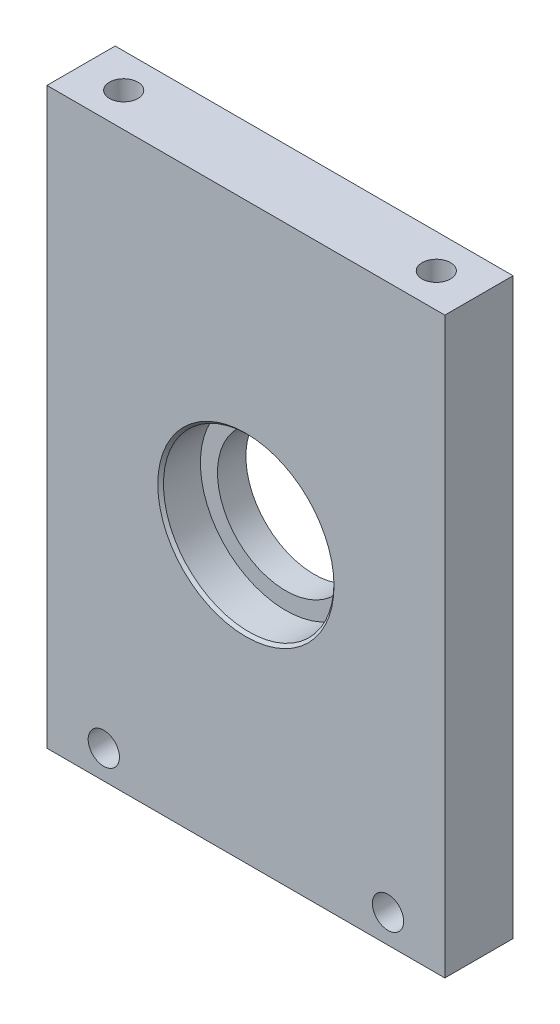
SolidWorks part; units mm, degrees
ref_plane "前视" through (0, 0, 0) normal (0, 0, 1) x (1, 0, 0)
ref_plane "上视" through (0, 0, 0) normal (0, 1, 0) x (1, 0, 0)
ref_plane "右视" through (0, 0, 0) normal (1, 0, 0) x (0, 0, -1)
sketch "草图1" plane through (0, 0, 0) normal (0, 0, 1) x (1, 0, 0)
  line L1 (0, 0) -> (70, 0)
  line L2 (0, 0) -> (0, -101)
  line L3 (0, -101) -> (70, -101)
  line L4 (70, 0) -> (70, -101)
  dimension "D1" = 70
  dimension "D2" = 101
extrude "凸台-拉伸1" add sketch "草图1" along normal blind 12
sketch "草图2" plane through (0, 0, 12) normal (0, 0, 1) x (1, 0, 0)
  line L0 (35, -51) -> (35, -101) construction
  line L1 (0, -101) -> (70, -101) construction
  circle A0 centre (35, -51) radius 15
  dimension "D1" = 30
  dimension "D2" = 50
extrude "切除-拉伸1" cut sketch "草图2" against normal blind 7
sketch "草图3" plane through (0, 0, 5) normal (0, 0, 1) x (1, 0, 0)
  circle A0 centre (35, -51) radius 12
  dimension "D1" = 24
extrude "切除-拉伸2" cut sketch "草图3" against normal through all
chamfer "倒角2" distance 0.5 angle 45 1 edges at (50, -51, 12)
hole_wizard "M6 螺纹孔1" positions "草图5" profile "草图4" tap size "M6" standard "GB"
sketch "草图5" plane through (0, 0, 0) normal (0, 1, 0) x (1, 0, 0)
  line L0 (62.5, -6) -> (7.5, -6) construction
  line L3 (35, -6) -> (35, -12) construction
  line L4 (70, -12) -> (0, -12) construction
  point P0 (62.5, -6)
  point P2 (7.5, -6)
  dimension "D1" = 6
  dimension "D2" = 55
sketch "草图4" plane through (62.5, 0, 6) normal (1, 0, 0) x (0, 0, 1)
  line L0 (0, 0) -> (0, 18.5022)
  line L1 (0, 18.5022) -> (2.5, 17)
  line L2 (2.5, 17) -> (2.5, 0)
  line L5 (2.5, 0) -> (0, 0)
  line L10 (0, 18.5022) -> (-2.5, 17) construction
  line L11 (0, -6.35) -> (0, 107.95) construction
  dimension "螺纹孔钻头直径" = 5
  dimension "螺纹孔钻头深度" = 17
  dimension "导头角度" = 118
cosmetic thread "孔螺蚊线1" parameters "D1"=12, "D2"=6
cosmetic thread "孔螺蚊线2" parameters "D1"=12, "D2"=6
sketch "草图10" plane through (0, 0, 0) normal (0, 0, -1) x (-1, 0, 0)
  line L0 (-60, -96) -> (-10, -96) construction
  line L1 (-35, -96) -> (-35, -101) construction
  line L2 (0, -101) -> (-70, -101) construction
  circle A0 centre (-60, -96) radius 2.75
  circle A1 centre (-10, -96) radius 2.75
  dimension "D3" = 5.5
  dimension "D1" = 5
  dimension "D2" = 50
extrude "切除-拉伸3" cut sketch "草图10" against normal through all
